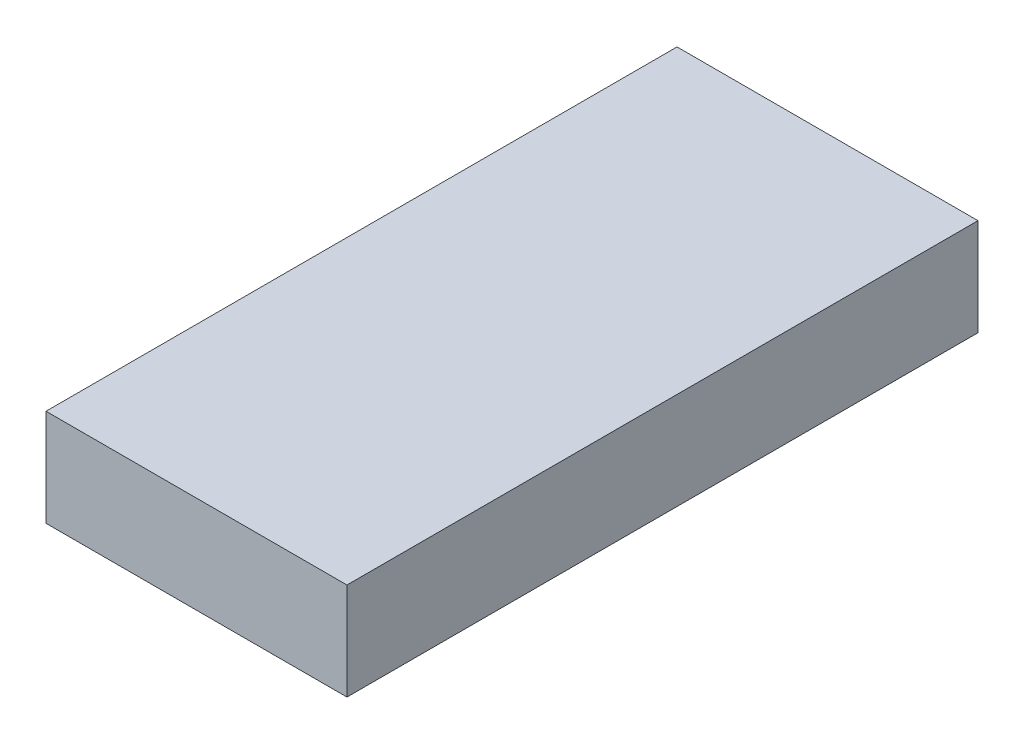
SolidWorks part; units mm, degrees
material "标准件"
ref_plane "前视基准面" through (0, 0, 0) normal (0, 0, 1) x (1, 0, 0)
ref_plane "上视基准面" through (0, 0, 0) normal (0, 1, 0) x (1, 0, 0)
ref_plane "右视基准面" through (0, 0, 0) normal (1, 0, 0) x (0, 0, -1)
sketch "草图1" plane through (0, 0, 0) normal (0, 1, 0) x (1, 0, 0)
  line L1 (-155, -325) -> (155, -325)
  line L2 (-155, -325) -> (-155, 325)
  line L3 (-155, 325) -> (155, 325)
  line L4 (155, -325) -> (155, 325)
  line L5 (-155, -325) -> (155, 325) construction
  line L6 (-155, 325) -> (155, -325) construction
  point P0 (0, 0)
  dimension "D1" = 650
  dimension "D2" = 310
extrude "凸台-拉伸1" add sketch "草图1" along normal blind 100
